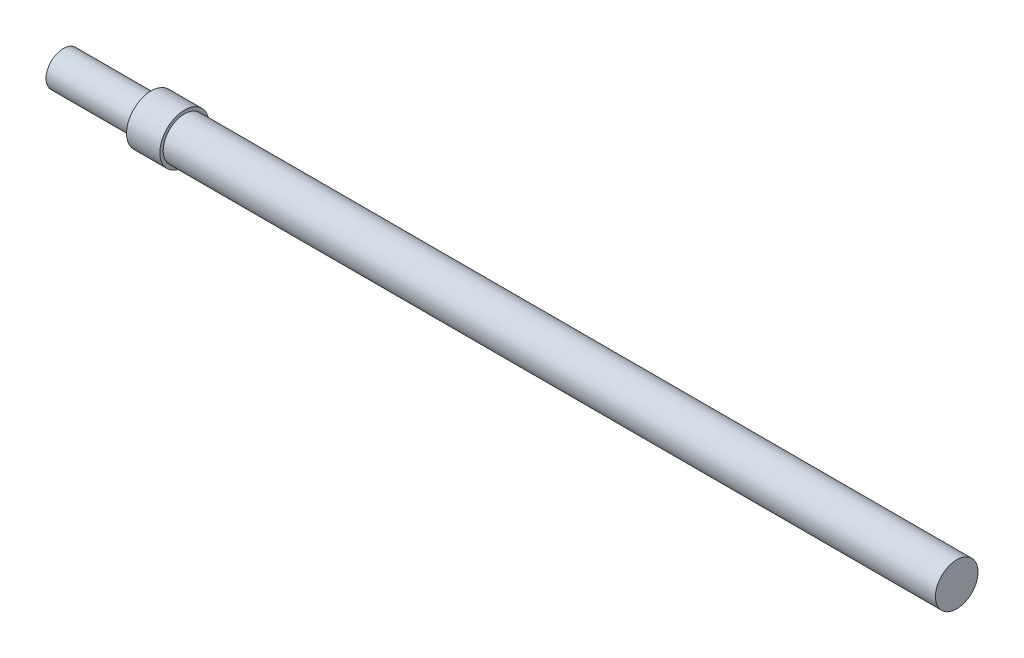
from build123d import *


with BuildPart() as part:
    # 草图1 → 旋转1 (revolve)
    with BuildSketch(Plane.XY, mode=Mode.PRIVATE) as revolve_1_sk:
        Polygon((-81.397540736, 0), (-81.397540736, 13), (-15.397540736, 13), (-15.397540736, 18.5), (9.602459264, 18.5), (9.602459264, 16), (589.602459264, 16), (589.602459264, 0), align=None)
    revolve(revolve_1_sk.sketch.rotate(Axis((-87.302640715, 0, 0), (1, 0, 0)), 90), axis=Axis((-87.302640715, 0, 0), (1, 0, 0)))


solid = part.part
